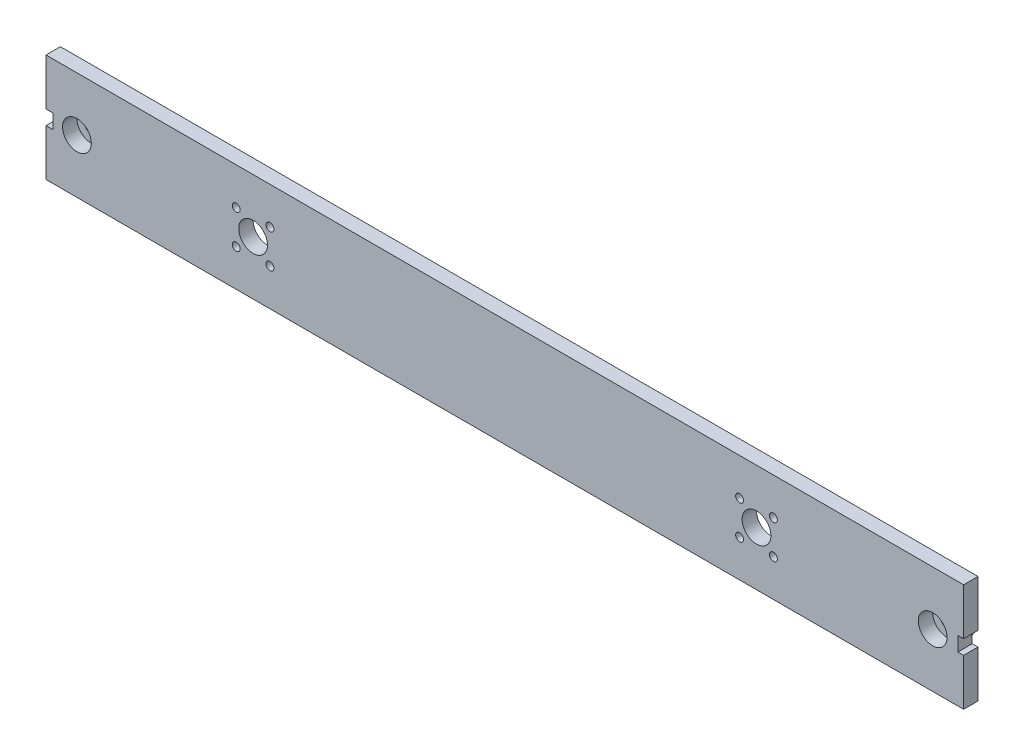
from build123d import *

# Parameters (mm, degrees)
SKETCH1_W             = 1276
SKETCH1_H             = 150
SKETCH1_R             = 20
SKETCH1_R_2           = 3.5
BOSS_EXTRUDE1_DEPTH   = 20
SKETCH2_R             = 5.5
CUT_EXTRUDE1_DEPTH    = 9
SKETCH4_W             = 20
SKETCH4_H             = 20
SKETCH4_W_2           = 16
CUT_EXTRUDE2_DEPTH    = 1285.942022038
SKETCH5_R             = 20
CUT_EXTRUDE3_DEPTH    = 1285.942022038
SKETCH6_R             = 25
SKETCH6_R_2           = 9
BOSS_EXTRUDE2_DEPTH   = 14
BOSS_EXTRUDE2_2_DEPTH = 14


with BuildPart() as part:
    # Sketch1 → Boss-Extrude1 (new body)
    with BuildSketch(Plane.XY):
        with Locations((638, 75)):
            Rectangle(SKETCH1_W, SKETCH1_H)
        with Locations((288, 75)):
            Circle(SKETCH1_R, mode=Mode.SUBTRACT)
        with Locations((264.5, 98.5)):
            Circle(SKETCH1_R_2, mode=Mode.SUBTRACT)
        with Locations((311.5, 98.5)):
            Circle(SKETCH1_R_2, mode=Mode.SUBTRACT)
        with Locations((311.5, 51.5)):
            Circle(SKETCH1_R_2, mode=Mode.SUBTRACT)
        with Locations((264.5, 51.5)):
            Circle(SKETCH1_R_2, mode=Mode.SUBTRACT)
        with Locations(Location((964.5, 51.5, 0), (0, 0, 180))):
            Circle(SKETCH1_R_2, mode=Mode.SUBTRACT)
        with Locations(Location((1011.5, 51.5, 0), (0, 0, 180))):
            Circle(SKETCH1_R_2, mode=Mode.SUBTRACT)
        with Locations(Location((988, 75, 0), (0, 0, 180))):
            Circle(SKETCH1_R, mode=Mode.SUBTRACT)
        with Locations(Location((1011.5, 98.5, 0), (0, 0, 180))):
            Circle(SKETCH1_R_2, mode=Mode.SUBTRACT)
        with Locations(Location((964.5, 98.5, 0), (0, 0, 180))):
            Circle(SKETCH1_R_2, mode=Mode.SUBTRACT)
    extrude(amount=BOSS_EXTRUDE1_DEPTH)

    # Sketch2 → Cut-Extrude1 (cut)
    with BuildSketch(Plane.XY.offset(20)):
        with Locations((264.5, 98.5)):
            Circle(SKETCH2_R)
        with Locations((311.5, 98.5)):
            Circle(SKETCH2_R)
        with Locations((311.5, 51.5)):
            Circle(SKETCH2_R)
        with Locations((264.5, 51.5)):
            Circle(SKETCH2_R)
        with Locations((964.5, 98.5)):
            Circle(SKETCH2_R)
        with Locations((1011.5, 98.5)):
            Circle(SKETCH2_R)
        with Locations((1011.5, 51.5)):
            Circle(SKETCH2_R)
        with Locations((964.5, 51.5)):
            Circle(SKETCH2_R)
    extrude(amount=-CUT_EXTRUDE1_DEPTH, mode=Mode.SUBTRACT)

    # Sketch4 → Cut-Extrude2 (cut, through all)
    with BuildSketch(Plane.XY.offset(20)):
        with Locations((0, 75)):
            Rectangle(SKETCH4_W, SKETCH4_H)
        with Locations((1276, 75)):
            Rectangle(SKETCH4_W_2, SKETCH4_H)
    extrude(amount=-CUT_EXTRUDE2_DEPTH, mode=Mode.SUBTRACT)

    # Sketch5 → Cut-Extrude3 (cut, through all)
    with BuildSketch(Plane.XY.offset(20)):
        with Locations((43, 75)):
            Circle(SKETCH5_R)
        with Locations((1233, 75)):
            Circle(SKETCH5_R)
    extrude(amount=-CUT_EXTRUDE3_DEPTH, mode=Mode.SUBTRACT)


with BuildPart() as body_2:
    # Sketch6 → Boss-Extrude2 (new body)
    with BuildSketch(Plane.XY):
        with Locations((43, 75)):
            Circle(SKETCH6_R)
        with Locations((43, 75)):
            Circle(SKETCH6_R_2, mode=Mode.SUBTRACT)
    extrude(amount=-BOSS_EXTRUDE2_DEPTH)


with BuildPart() as body_3:
    # Sketch6 → Boss-Extrude2 2 (new body)
    with BuildSketch(Plane.XY):
        with Locations((1233, 75)):
            Circle(SKETCH6_R)
        with Locations((1233, 75)):
            Circle(SKETCH6_R_2, mode=Mode.SUBTRACT)
    extrude(amount=-BOSS_EXTRUDE2_2_DEPTH)


solid = Compound([part.part, body_2.part, body_3.part])
